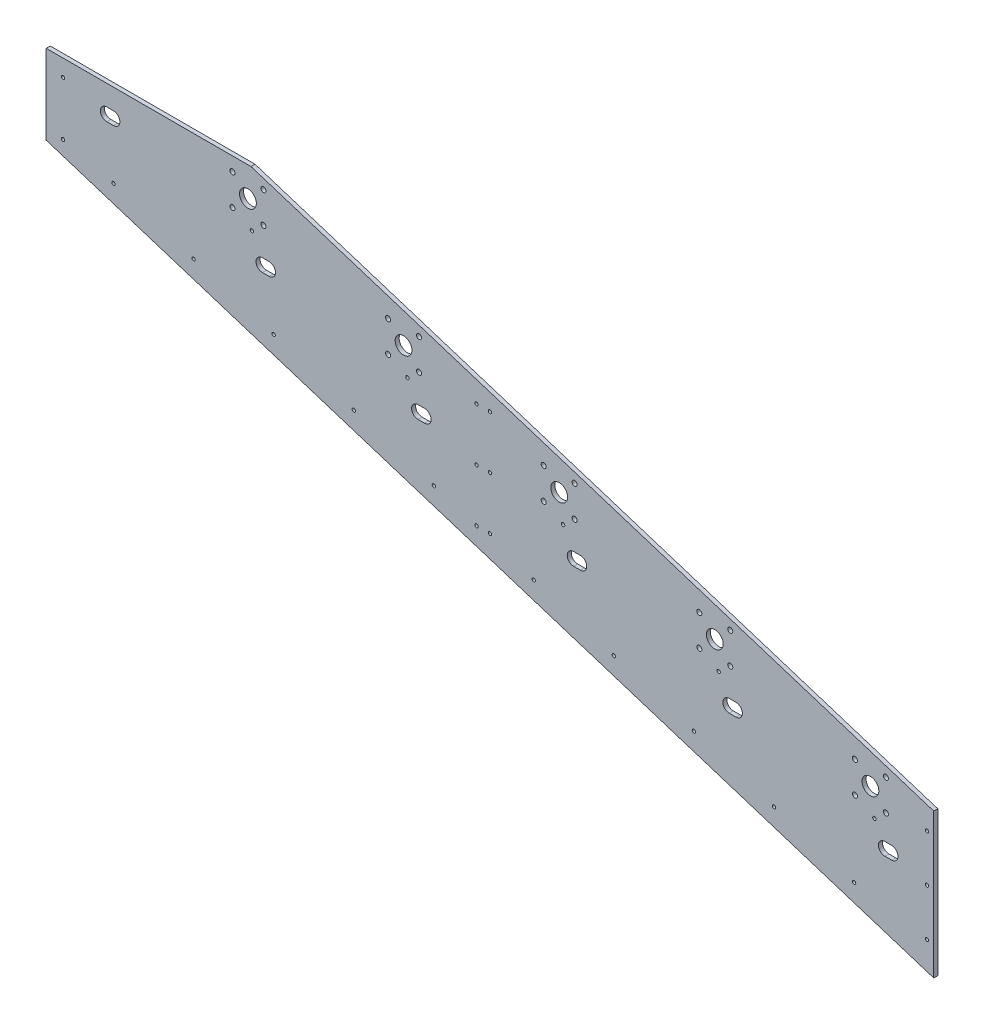
SolidWorks part; units mm, degrees
ref_plane "前视基准面" through (0, 0, 0) normal (0, 0, 1) x (1, 0, 0)
ref_plane "上视基准面" through (0, 0, 0) normal (0, 1, 0) x (1, 0, 0)
ref_plane "右视基准面" through (0, 0, 0) normal (1, 0, 0) x (0, 0, -1)
sketch "草图1" plane through (0, 0, -510) normal (0, 0, 1) x (1, 0, 0)
  line L0 (3700, 0) -> (3700, 565.3394) construction
  line L1 (0, 1611) -> (3700, 1611)
  line L2 (0, 1611) -> (0, 435)
  line L3 (0, 435) -> (3700, 435)
  line L4 (3700, 1611) -> (3700, 435)
  line L5 (3600, 435) -> (100, 435) construction
extrude "凸台-拉伸1" add sketch "草图1" along normal blind 12
sketch "草图2" plane through (0, 0, -510) normal (0, 0, -1) x (-1, 0, 0)
  line L0 (-3700, 1611) -> (0, 1611) construction
  line L2 (-100, 1611) -> (-100, 1447.3384) construction
  line L3 (-200, 1531) -> (-778.7469, 1531) construction
  line L4 (-200, 1531) -> (-599.9391, 1524.019) construction
  circle A0 centre (-200, 1531) radius 19
  circle A1 centre (-599.9391, 1524.019) radius 25
  dimension "D1" = 38
  dimension "D2" = 50
  dimension "D3" = 80
  dimension "D4" = 100
  dimension "D5" = 1
  dimension "D6" = 400
extrude "切除-拉伸1" cut sketch "草图2" against normal through all
sketch "草图3" plane through (0, 0, -510) normal (0, 0, -1) x (-1, 0, 0)
  line L0 (-200, 1531) -> (-662.9391, 1384.019)
  point P0 (-662.9391, 1384.019)
  point P1 (-599.9391, 1524.019)
  dimension "D1" = 63
  dimension "D2" = 140
pattern_linear "阵列(线性)1" count 5 spacing 485.7118 along (0.9531, -0.3026, 0) of "切除-拉伸1"
sketch "草图5" plane through (0, 0, -510) normal (0, 0, -1) x (-1, 0, 0)
  line L0 (-608.9458, 1611) -> (-3700, 629.6049)
  line L1 (-3700, 1611) -> (0, 1611) construction
  line L2 (-3700, 435) -> (-3700, 1611) construction
  line L3 (-200, 1531) -> (-662.9391, 1384.019) construction
  line L4 (-3700, 629.6049) -> (-3700, 1611)
  line L5 (-3700, 1611) -> (-608.9458, 1611)
  dimension "D1" = 200
extrude "切除-拉伸2" cut sketch "草图5" against normal through all
sketch "草图6" plane through (0, 0, -510) normal (0, 0, -1) x (-1, 0, 0)
  line L0 (-2958.0561, 435) -> (0, 1374.1688)
  line L2 (0, 1611) -> (0, 435) construction
  line L3 (-200, 1531) -> (-662.9391, 1384.019) construction
  line L4 (0, 1374.1688) -> (0, 435)
  line L6 (0, 435) -> (-2958.0561, 435)
  line L7 (-3600, 435) -> (-100, 435) construction
  line L9 (0, 1611) -> (0, 0) construction
  dimension "D1" = 210
extrude "切除-拉伸4" cut sketch "草图6" against normal through all
sketch "草图7" plane through (0, 0, -510) normal (0, 0, -1) x (-1, 0, 0)
  line L0 (-200, 1531) -> (-180, 1531) construction
  line L1 (-200, 1550) -> (-180, 1550)
  line L2 (-200, 1512) -> (-180, 1512)
  arc A0 (-200, 1550) -> (-200, 1512) centre (-200, 1531) ccw
  arc A1 (-180, 1512) -> (-180, 1550) centre (-180, 1531) ccw
  circle A2 centre (-200, 1531) radius 19 construction
  point P3 (-190, 1531)
  dimension "D1" = 20
extrude "切除-拉伸5" cut sketch "草图7" against normal through all
pattern_linear "阵列(线性)2" count 6 spacing 485.7118 along (0.9531, -0.3026, 0) of "切除-拉伸5"
sketch "草图9" plane through (0, 0, -510) normal (0, 0, -1) x (-1, 0, 0)
  circle A0 centre (-553.9391, 1570.019) radius 7.5
  circle A1 centre (-645.9391, 1570.019) radius 7.5
  circle A2 centre (-645.9391, 1478.019) radius 7.5
  circle A3 centre (-553.9391, 1478.019) radius 7.5
  dimension "D1" = 15
extrude "切除-拉伸11" cut sketch "草图9" against normal through all
sketch "草图10" plane through (0, 0, -510) normal (0, 0, -1) x (-1, 0, 0)
  line L0 (-599.9391, 1524.019) -> (-599.9391, 1667.1464) construction
  line L1 (-599.9391, 1524.019) -> (-602.0857, 1647.0003) construction
  circle A0 centre (-602.0857, 1647.0003) radius 25
  dimension "D1" = 1
  dimension "D2" = 123
  dimension "D3" = 50
sketch "草图11" plane through (0, 0, -510) normal (0, 0, -1) x (-1, 0, 0)
  circle A0 centre (-50, 1561) radius 5 construction
  circle A1 centre (-50, 1401) radius 5 construction
  circle A2 centre (-200, 1363.1293) radius 5 construction
  circle A3 centre (-438.2787, 1287.477) radius 5 construction
  circle A4 centre (-676.5573, 1211.8246) radius 5 construction
  circle A5 centre (-914.836, 1136.1723) radius 5 construction
  circle A6 centre (-1153.1147, 1060.5199) radius 5 construction
  circle A7 centre (-1280, 1021) radius 5 construction
  circle A8 centre (-1320, 1021) radius 5 construction
  circle A9 centre (-1280, 1178) radius 5 construction
  circle A10 centre (-1320, 1178) radius 5 construction
  circle A11 centre (-1320, 1335) radius 5 construction
  circle A12 centre (-1280, 1335) radius 5 construction
  circle A13 centre (-1450, 966.2603) radius 5 construction
  circle A14 centre (-1688.2787, 890.6079) radius 5 construction
  circle A15 centre (-1926.5573, 814.9556) radius 5 construction
  circle A16 centre (-2164.836, 739.3032) radius 5 construction
  circle A17 centre (-2620, 625) radius 5 construction
  circle A19 centre (-2620, 765) radius 5 construction
  circle A22 centre (-2620, 905) radius 5 construction
  circle A23 centre (-2403.1147, 663.6509) radius 5 construction
  circle A24 centre (-2403.1147, 663.6509) radius 5
  circle A30 centre (-50, 1561) radius 5
  circle A31 centre (-50, 1401) radius 5
  circle A32 centre (-200, 1363.1293) radius 5
  circle A33 centre (-438.2787, 1287.477) radius 5
  circle A34 centre (-676.5573, 1211.8246) radius 5
  circle A35 centre (-914.836, 1136.1723) radius 5
  circle A36 centre (-1153.1147, 1060.5199) radius 5
  circle A37 centre (-1280, 1021) radius 5
  circle A38 centre (-1320, 1021) radius 5
  circle A39 centre (-1280, 1178) radius 5
  circle A40 centre (-1320, 1178) radius 5
  circle A41 centre (-1320, 1335) radius 5
  circle A42 centre (-1280, 1335) radius 5
  circle A43 centre (-1450, 966.2603) radius 5
  circle A44 centre (-1688.2787, 890.6079) radius 5
  circle A45 centre (-1926.5573, 814.9556) radius 5
  circle A46 centre (-2164.836, 739.3032) radius 5
  circle A47 centre (-2620, 625) radius 5
  circle A49 centre (-2620, 765) radius 5
  circle A52 centre (-2620, 905) radius 5
extrude "切除-拉伸12" cut sketch "草图11" against normal through all
ref_plane "基准面1" through (1300, 0, 0) normal (-1, 0, 0) x (0, 0, 1)
ref_plane "基准面2" through (2640, 0, 0) normal (-1, 0, 0) x (0, 0, 1)
pattern_linear "阵列(线性)3" count 5 spacing 485.7118 along (0.9531, -0.3026, 0) of "切除-拉伸11"
other "使用曲面切除1"
sketch "草图12" plane through (0, 0, -510) normal (0, 0, -1) x (-1, 0, 0)
  circle A0 centre (-611.6791, 1446.789) radius 5
  dimension "D1" = 10
  dimension "D2" = 77.23
  dimension "D3" = 11.74
extrude "切除-拉伸13" cut sketch "草图12" against normal through all
pattern_linear "阵列(线性)4" count 5 spacing 485.7118 along (0.9531, -0.3026, 0) of "切除-拉伸13"
sketch "草图14" plane through (0, 0, -510) normal (0, 0, -1) x (-1, 0, 0)
  line L0 (-662.9391, 1365.019) -> (-642.9391, 1365.019) construction
  line L1 (-642.9391, 1403.019) -> (-662.9391, 1403.019) construction
  line L2 (-662.9391, 1365.019) -> (-642.9391, 1365.019) construction
  line L3 (-642.9391, 1403.019) -> (-662.9391, 1403.019) construction
  line L4 (-662.9391, 1384.019) -> (-662.9391, 1374.019) construction
  line L5 (-642.9391, 1393.019) -> (-662.9391, 1393.019)
  line L6 (-662.9391, 1355.019) -> (-642.9391, 1355.019)
  arc A0 (-642.9391, 1365.019) -> (-642.9391, 1403.019) centre (-642.9391, 1384.019) ccw construction
  arc A1 (-662.9391, 1403.019) -> (-662.9391, 1365.019) centre (-662.9391, 1384.019) ccw construction
  arc A2 (-642.9391, 1365.019) -> (-642.9391, 1403.019) centre (-642.9391, 1384.019) ccw construction
  arc A3 (-662.9391, 1403.019) -> (-662.9391, 1365.019) centre (-662.9391, 1384.019) ccw construction
  arc A4 (-662.9391, 1393.019) -> (-662.9391, 1355.019) centre (-662.9391, 1374.019) ccw
  arc A5 (-642.9391, 1355.019) -> (-642.9391, 1393.019) centre (-642.9391, 1374.019) ccw
  dimension "D1" = 10
  dimension "D2" = 2
sketch "草图15" plane through (0, 0, -510) normal (0, 0, -1) x (-1, 0, 0)
  line L0 (-662.9391, 1384.019) -> (-642.9391, 1384.019) construction
  line L1 (-662.9391, 1414.019) -> (-642.9391, 1414.019)
  line L2 (-662.9391, 1354.019) -> (-642.9391, 1354.019)
  line L3 (-1125.8782, 1237.0381) -> (-1105.8782, 1237.0381) construction
  line L4 (-1125.8782, 1267.0381) -> (-1105.8782, 1267.0381)
  line L5 (-1125.8782, 1207.0381) -> (-1105.8782, 1207.0381)
  line L6 (-1588.8172, 1090.0571) -> (-1568.8172, 1090.0571) construction
  line L7 (-1588.8172, 1120.0571) -> (-1568.8172, 1120.0571)
  line L8 (-1588.8172, 1060.0571) -> (-1568.8172, 1060.0571)
  line L9 (-2051.7563, 943.0761) -> (-2031.7563, 943.0761) construction
  line L10 (-2051.7563, 973.0761) -> (-2031.7563, 973.0761)
  line L11 (-2051.7563, 913.0761) -> (-2031.7563, 913.0761)
  arc A0 (-662.9391, 1414.019) -> (-662.9391, 1354.019) centre (-662.9391, 1384.019) ccw
  arc A1 (-642.9391, 1354.019) -> (-642.9391, 1414.019) centre (-642.9391, 1384.019) ccw
  arc A2 (-1125.8782, 1267.0381) -> (-1125.8782, 1207.0381) centre (-1125.8782, 1237.0381) ccw
  arc A3 (-1105.8782, 1207.0381) -> (-1105.8782, 1267.0381) centre (-1105.8782, 1237.0381) ccw
  arc A4 (-1588.8172, 1120.0571) -> (-1588.8172, 1060.0571) centre (-1588.8172, 1090.0571) ccw
  arc A5 (-1568.8172, 1060.0571) -> (-1568.8172, 1120.0571) centre (-1568.8172, 1090.0571) ccw
  arc A6 (-2051.7563, 973.0761) -> (-2051.7563, 913.0761) centre (-2051.7563, 943.0761) ccw
  arc A7 (-2031.7563, 913.0761) -> (-2031.7563, 973.0761) centre (-2031.7563, 943.0761) ccw
  point P4 (-652.9391, 1384.019)
  point P13 (-1115.8782, 1237.0381)
  point P22 (-1578.8172, 1090.0571)
  point P31 (-2041.7563, 943.0761)
  dimension "D1" = 30
extrude "凸台-拉伸4" add sketch "草图15" against normal through all
extrude "切除-拉伸14" cut sketch "草图14" against normal through all contours A5 L5 A4 L6
pattern_linear "阵列(线性)5" count 4 spacing 485.7118 along (0.9531, -0.3026, 0) of "切除-拉伸14"
equation "\"b1\"= \"RD1@注解\""
equation "\"D3@阵列(线性)1\"=\"b1\""
equation "\"D3@阵列(线性)2\"=\"b1\""
equation "\"D3@阵列(线性)3\"=\"b1\""
equation "\"D3@阵列(线性)4\"=\"b1\""
equation "\"D3@阵列(线性)5\"=\"b1\""
